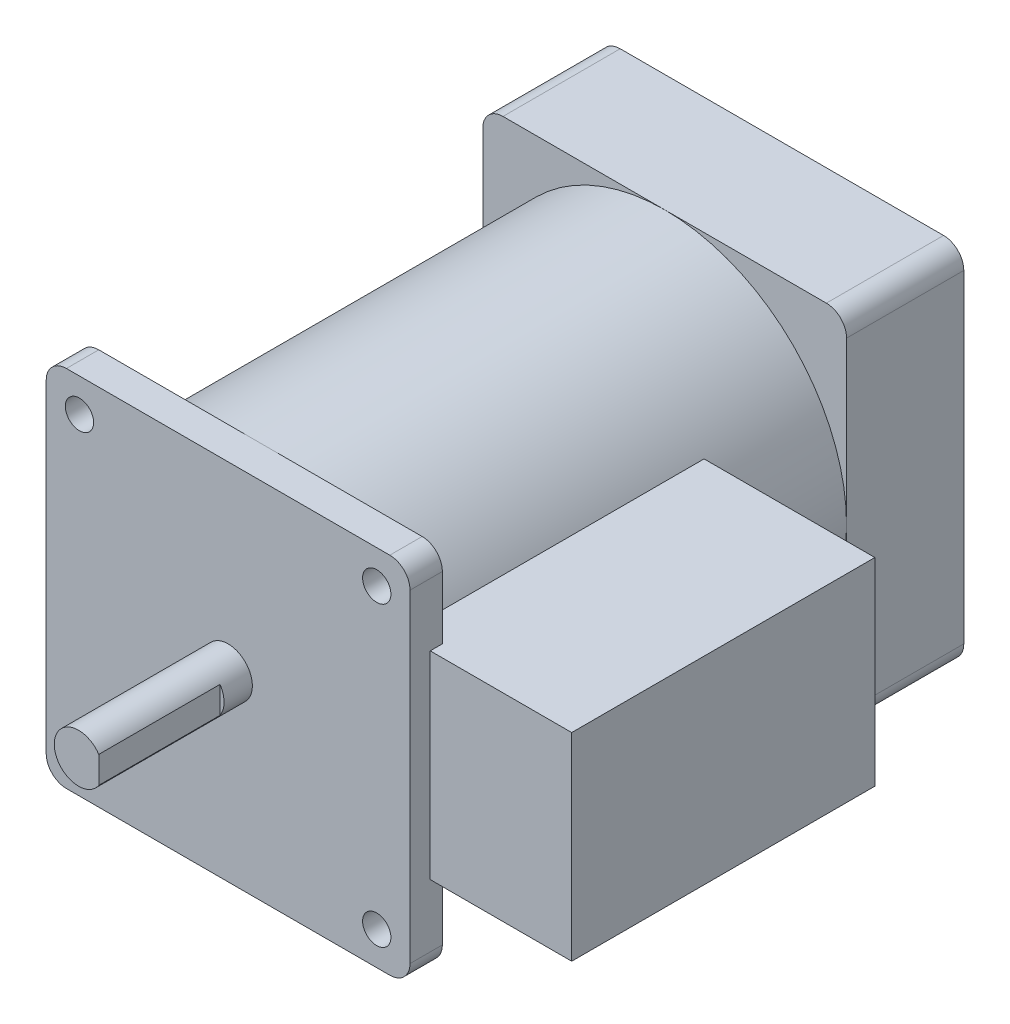
SolidWorks part; units mm, degrees
ref_plane "前视基准面" through (0, 0, 0) normal (0, 0, 1) x (1, 0, 0)
ref_plane "上视基准面" through (0, 0, 0) normal (0, 1, 0) x (1, 0, 0)
ref_plane "右视基准面" through (0, 0, 0) normal (1, 0, 0) x (0, 0, -1)
sketch "草图1" plane through (0, 0, 0) normal (0, 0, 1) x (1, 0, 0)
  line L0 (0, 45) -> (0, 0) construction
  line L1 (-45, 45) -> (45, 45)
  line L2 (-45, 45) -> (-45, -45)
  line L3 (-45, -45) -> (45, -45)
  line L4 (45, 45) -> (45, -45)
  line L5 (0, 0) -> (45, 0) construction
  dimension "D1" = 90
  dimension "D2" = 90
extrude "凸台-拉伸1" add sketch "草图1" along normal blind 8
sketch "草图2" plane through (0, 0, 0) normal (0, 0, -1) x (-1, 0, 0)
  circle A0 centre (0, 0) radius 45
  dimension "D1" = 90
extrude "凸台-拉伸2" add sketch "草图2" along normal blind 100
sketch "草图3" plane through (0, 0, -100) normal (0, 0, -1) x (-1, 0, 0)
  line L0 (0, 22.5569) -> (0, 0) construction
  line L1 (-45, 45) -> (45, 45)
  line L2 (-45, 45) -> (-45, -45)
  line L3 (-45, -45) -> (45, -45)
  line L4 (45, 45) -> (45, -45)
  line L5 (0, 0) -> (61.1832, 0) construction
  dimension "D1" = 90
  dimension "D2" = 90
extrude "凸台-拉伸3" add sketch "草图3" along normal blind 29
sketch "草图4" plane through (0, 0, 8) normal (0, 0, 1) x (1, 0, 0)
  circle A0 centre (0, 0) radius 6
  dimension "D1" = 12
extrude "凸台-拉伸4" add sketch "草图4" along normal blind 37
sketch "草图6" plane through (0, 0, 0) normal (1, 0, 0) x (0, 0, -1)
  line L0 (0, 0) -> (45.1465, 0) construction
  line L1 (-3, 24.5) -> (72, 24.5)
  line L2 (-3, 24.5) -> (-3, -24.5)
  line L3 (-3, -24.5) -> (72, -24.5)
  line L4 (72, 24.5) -> (72, -24.5)
  line L5 (-8, -45) -> (-8, 45) construction
  dimension "D1" = 49
  dimension "D2" = 75
  dimension "D3" = 5
extrude "凸台-拉伸5" add sketch "草图6" along normal blind 80
sketch "草图7" plane through (0, 0, 8) normal (0, 0, 1) x (1, 0, 0)
  line L0 (0, 0) -> (0, 59.3172) construction
  line L1 (0, 0) -> (-27.2353, 27.2353) construction
  circle A0 centre (0, 0) radius 52 construction
  circle A1 centre (-36.7696, 36.7696) radius 3.5
  dimension "D1" = 104
  dimension "D2" = 7
  dimension "D3" = 45
extrude "切除-拉伸1" cut sketch "草图7" against normal up to surface (8 mm away) up to face at (-33.1066, 33.1066, 0)
fillet "圆角1" radius 5 4 edges at (45, -45, 4) (-45, -45, 4) (45, 45, 4) (-45, 45, 4)
fillet "圆角2" radius 5 4 edges at (45, -45, -114.5) (-45, -45, -114.5) (45, 45, -114.5) (-45, 45, -114.5)
ref_plane "基准面1" through (6, 0, 0) normal (1, 0, 0) x (0, 0, -1)
sketch "草图8" plane through (6, 0, 0) normal (1, 0, 0) x (0, 0, -1)
  line L0 (-45, 0) -> (-24.7845, 0) construction
  line L1 (-45, 2) -> (-15, 2)
  line L2 (-45, 2) -> (-45, -2)
  line L3 (-45, -2) -> (-15, -2)
  line L5 (-45, 6) -> (-45, -6) construction
  arc A0 (-15, -2) -> (-15, 2) centre (-15, 0) ccw
  dimension "D1" = 4
  dimension "D2" = 30
sketch "草图9" plane through (6, 0, 0) normal (1, 0, 0) x (0, 0, -1)
  line L0 (-45, 6) -> (-45, -6) construction
  line L1 (-45, 7.8842) -> (-15, 7.8842)
  line L2 (-45, 7.8842) -> (-45, -8.0535)
  line L3 (-45, -8.0535) -> (-15, -8.0535)
  line L4 (-15, 7.8842) -> (-15, -8.0535)
  dimension "D1" = 30
extrude "切除-拉伸2" cut sketch "草图9" against normal blind 1
pattern_circular "阵列(圆周)1" count 4 over 360 about axis through (0, 0, 0) along (0, 0, 1) of "切除-拉伸1"
